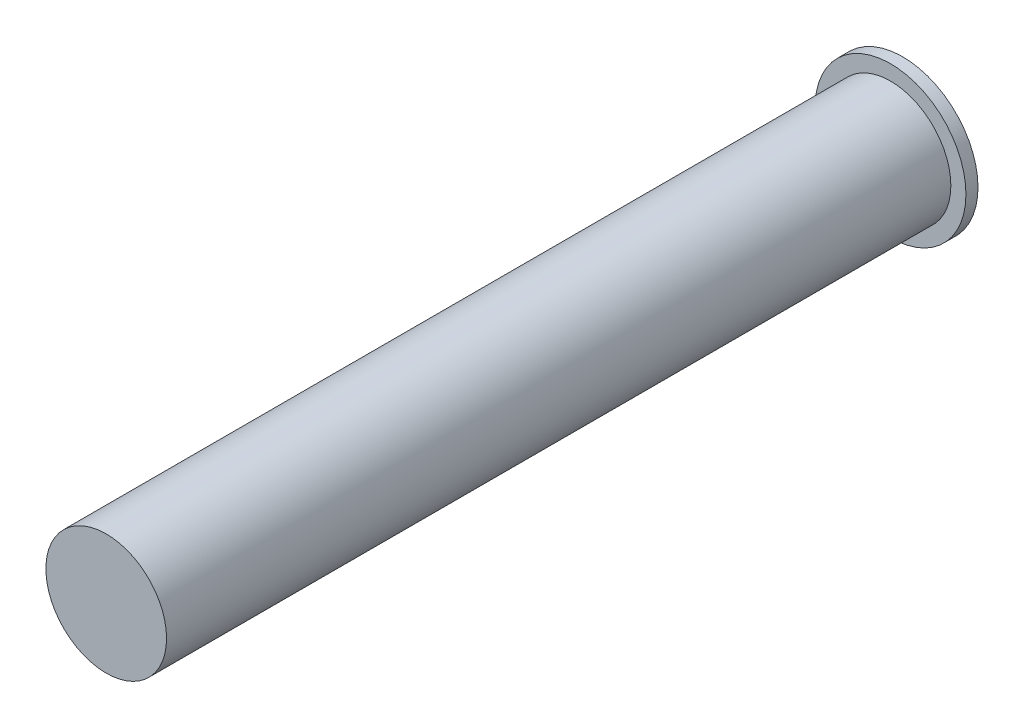
SolidWorks part; units mm, degrees
ref_plane "Front Plane" through (0, 0, 0) normal (0, 0, 1) x (1, 0, 0)
ref_plane "Top Plane" through (0, 0, 0) normal (0, 1, 0) x (1, 0, 0)
ref_plane "Right Plane" through (0, 0, 0) normal (1, 0, 0) x (0, 0, -1)
other "Configuration Table"
sketch "Sketch1" plane through (0, 0, 0) normal (0, 0, 1) x (1, 0, 0)
  circle A0 centre (0, 0) radius 12.5
  dimension "D1" = 25
extrude "Boss-Extrude1" add sketch "Sketch1" along normal blind 2
sketch "Sketch2" plane through (0, 0, 2) normal (0, 0, 1) x (1, 0, 0)
  circle A0 centre (0, 0) radius 10
  dimension "D1" = 20
extrude "Boss-Extrude7" add sketch "Sketch2" along normal blind 130
cosmetic thread "Cosmetic Thread1" parameters "D1"=20, "D2"=17.294
